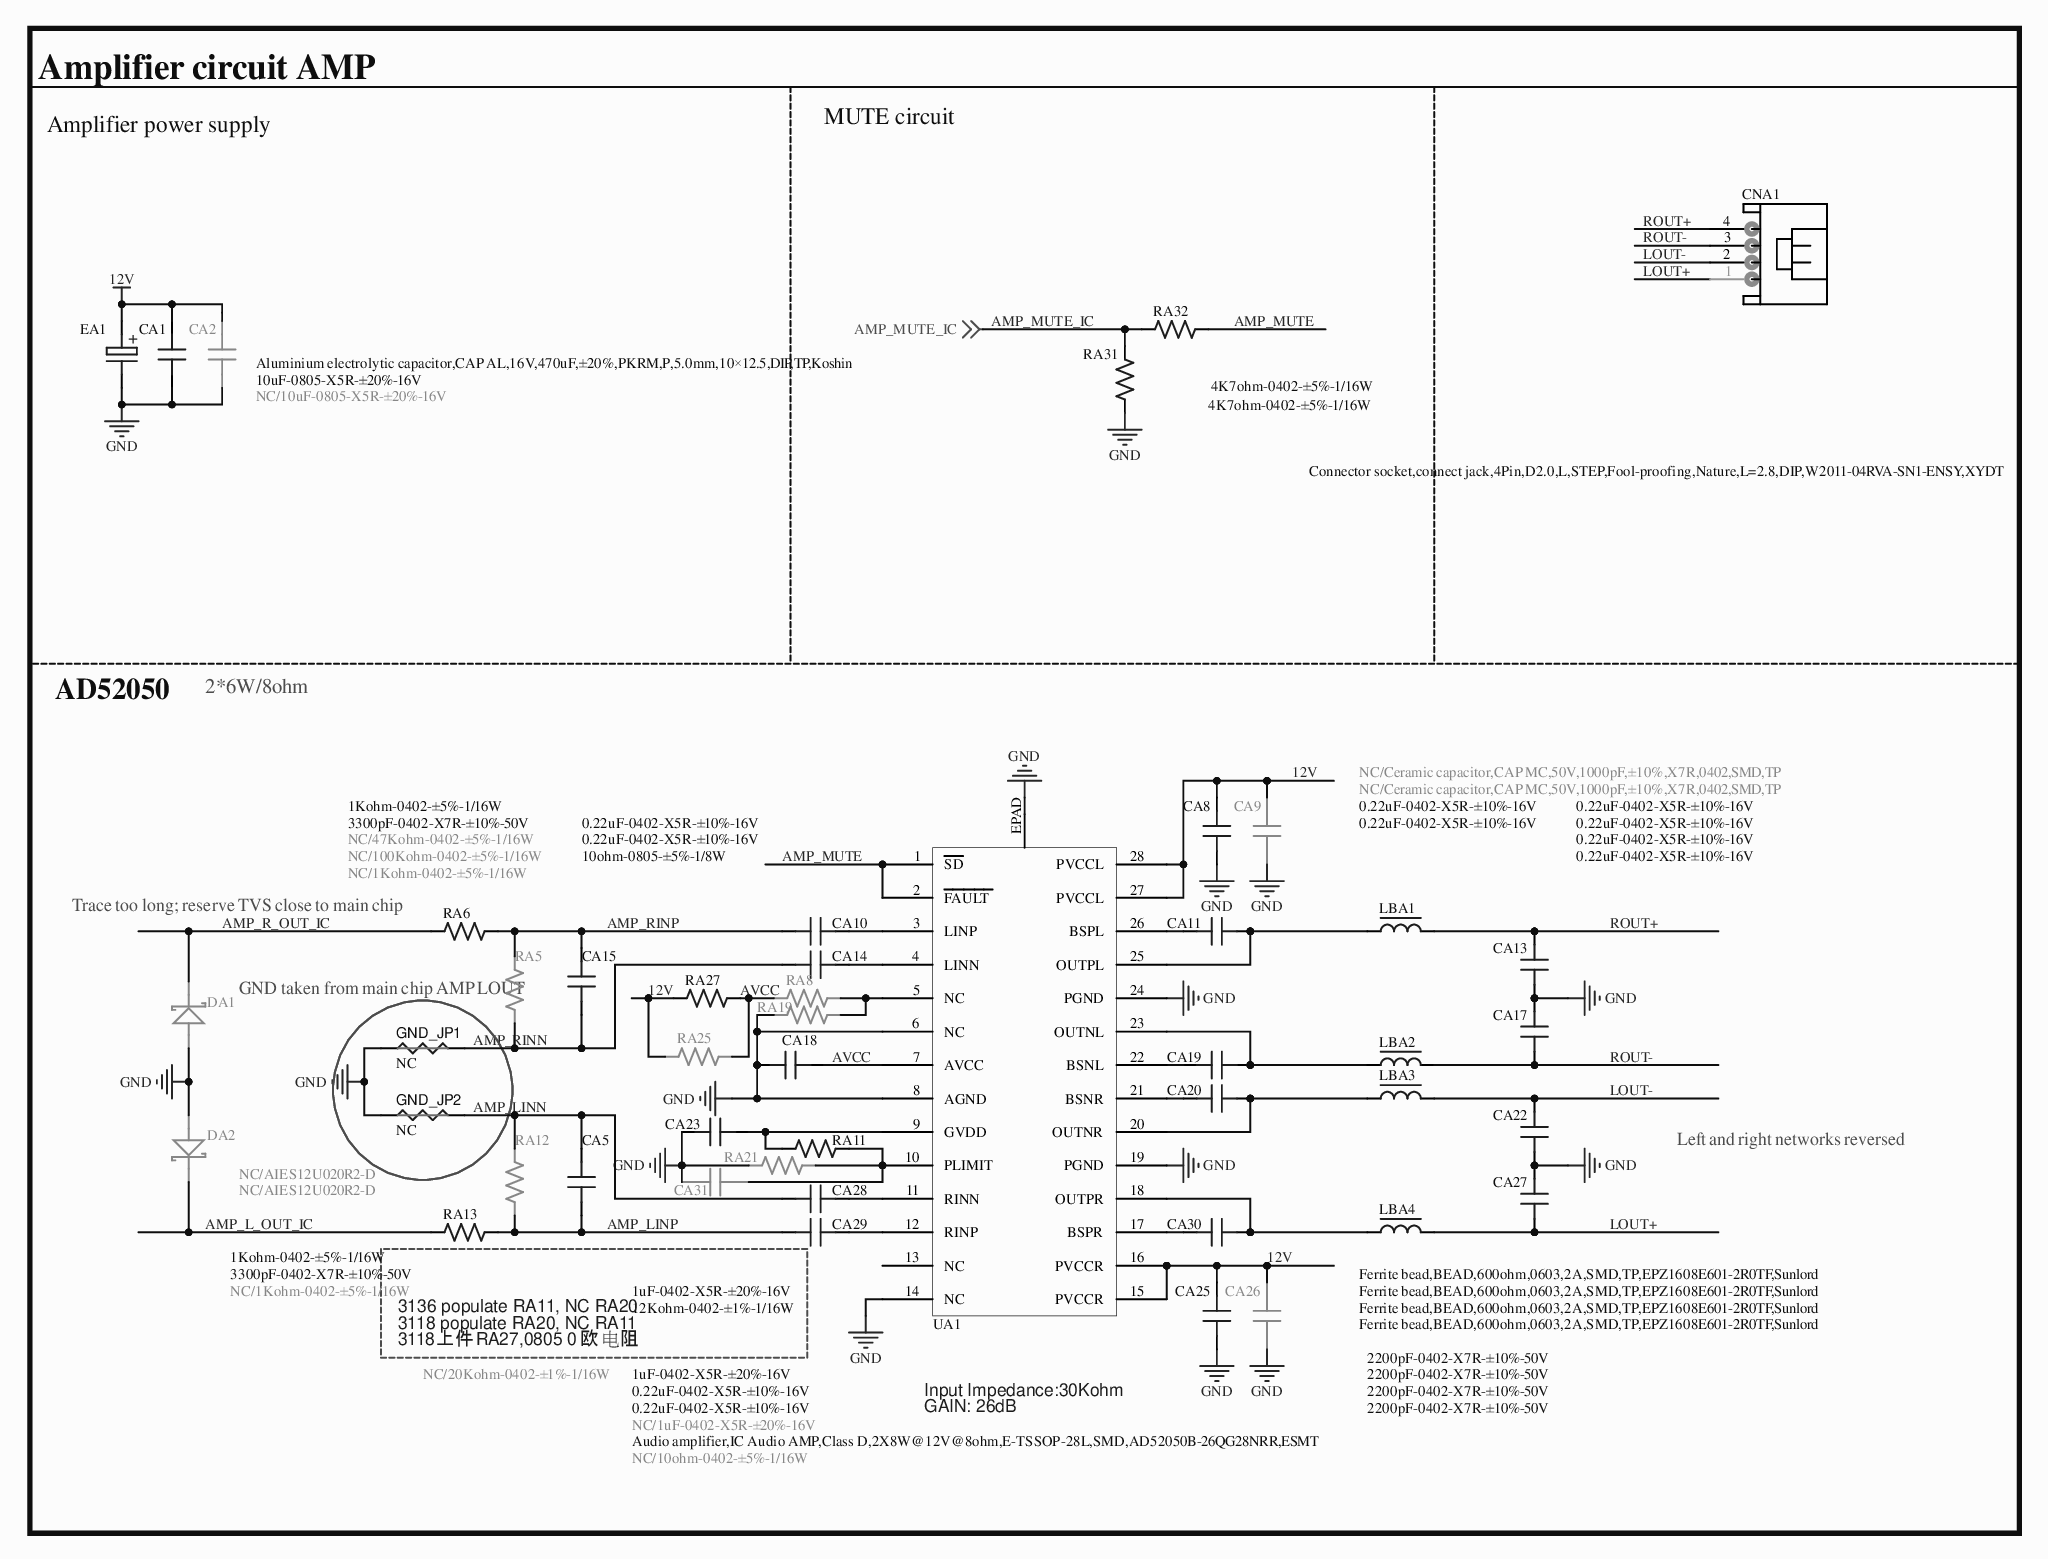
[diagram p0: MISC84395-16.SchDoc]
# Altium project MISC84395-37.PrjPCB (part 10 of 13)

## Sheet MISC84395-16.SchDoc
size 393 x 342 mm

### Parts
CA1  10uF-0805-X5R-±20%-16V  [C0805]
CA2  NC/10uF-0805-X5R-±20%-16V  [C0805]
CA5  3300pF-0402-X7R-±10%-50V  [C0402]
CA8  0.22uF-0402-X5R-±10%-16V  [C0402]
CA9  NC/Ceramic capacitor,CAP MC,50V,1000pF,±10%,X7R,0402,SMD,TP  [C0402]
CA10  0.22uF-0402-X5R-±10%-16V  [C0402]
CA11  0.22uF-0402-X5R-±10%-16V  [C0402]
CA13  2200pF-0402-X7R-±10%-50V  [C0402]
CA14  0.22uF-0402-X5R-±10%-16V  [C0402]
CA15  3300pF-0402-X7R-±10%-50V  [C0402]
CA17  2200pF-0402-X7R-±10%-50V  [C0402]
CA18  1uF-0402-X5R-±20%-16V  [C0402]
CA19  0.22uF-0402-X5R-±10%-16V  [C0402]
CA20  0.22uF-0402-X5R-±10%-16V  [C0402]
CA22  2200pF-0402-X7R-±10%-50V  [C0402]
CA23  1uF-0402-X5R-±20%-16V  [C0402]
CA25  0.22uF-0402-X5R-±10%-16V  [C0402]
CA26  NC/Ceramic capacitor,CAP MC,50V,1000pF,±10%,X7R,0402,SMD,TP  [C0402]
CA27  2200pF-0402-X7R-±10%-50V  [C0402]
CA28  0.22uF-0402-X5R-±10%-16V  [C0402]
CA29  0.22uF-0402-X5R-±10%-16V  [C0402]
CA30  0.22uF-0402-X5R-±10%-16V  [C0402]
CA31  NC/1uF-0402-X5R-±20%-16V  [C0402]
CNA1  Connector socket,connect jack,4Pin,D2.0,L,STEP,Fool-proofing,Nature,L=2.8,DIP,W2011-04RVA-SN1-ENSY,XYDT  [SIP4H/2.0D-6]
DA1  NC/AIES12U020R2-D  [DIODE-S0402]
DA2  NC/AIES12U020R2-D  [DIODE-S0402]
EA1  Aluminium electrolytic capacitor,CAP AL,16V,470uF,±20%,PKRM,P,5.0mm,10×12.5,DIP,TP,Koshin  [EC(10*12)-V-5]
GND_JP1  NC  [GND]
GND_JP2  NC  [GND]
LBA1  Ferrite bead,BEAD,600ohm,0603,2A,SMD,TP,EPZ1608E601-2R0TF,Sunlord  [L0603]
LBA2  Ferrite bead,BEAD,600ohm,0603,2A,SMD,TP,EPZ1608E601-2R0TF,Sunlord  [L0603]
LBA3  Ferrite bead,BEAD,600ohm,0603,2A,SMD,TP,EPZ1608E601-2R0TF,Sunlord  [L0603]
LBA4  Ferrite bead,BEAD,600ohm,0603,2A,SMD,TP,EPZ1608E601-2R0TF,Sunlord  [L0603]
RA5  NC/1Kohm-0402-±5%-1/16W  [R0402]
RA6  1Kohm-0402-±5%-1/16W  [R0402]
RA8  NC/100Kohm-0402-±5%-1/16W  [R0402]
RA11  12Kohm-0402-±1%-1/16W  [R0402]
RA12  NC/1Kohm-0402-±5%-1/16W  [R0402]
RA13  1Kohm-0402-±5%-1/16W  [R0402]
RA19  NC/47Kohm-0402-±5%-1/16W  [R0402]
RA21  NC/20Kohm-0402-±1%-1/16W  [R0402]
RA25  NC/10ohm-0402-±5%-1/16W  [R0402]
RA27  10ohm-0805-±5%-1/8W  [R0805]
RA31  4K7ohm-0402-±5%-1/16W  [R0402]
RA32  4K7ohm-0402-±5%-1/16W  [R0402]
UA1  Audio amplifier,IC Audio AMP,Class D,2X8W@12V@8ohm,E-TSSOP-28L,SMD,AD52050B-26QG28NRR,ESMT  [SOP28/0.65-7]

### Nets
12V: CA1.2 CA2.2 CA8.2 CA9.2 CA25.1 CA26.2 EA1.1 RA25.1 RA27.1 UA1.15(PVCCR) UA1.16(PVCCR) UA1.27(PVCCL) UA1.28(PVCCL)
GND: CA1.1 CA2.1 CA8.1 CA9.1 CA13.1 CA17.2 CA18.2 CA22.1 CA23.2 CA25.2 CA26.1 CA27.2 CA31.2 DA1.A DA2.A EA1.2 GND_JP1.JP_2K GND_JP2.JP_2K RA19.1 RA21.1 RA31.1 UA1.6(NC) UA1.8(AGND) UA1.14(NC) UA1.19(PGND) UA1.24(PGND) UA1.EPAD
AMP_L_OUT_IC: DA2.K RA13.1
AMP_LINN: CA5.2 CA28.2 GND_JP2.JP_1K RA12.2
AMP_LINP: CA5.1 CA29.2 RA12.1 RA13.2
AMP_MUTE: RA32.1 UA1.1(~{SD}) UA1.2(~{FAULT})
AMP_MUTE_IC: RA31.2 RA32.2 ; off-sheet AMP_MUTE_IC
AMP_R_OUT_IC: DA1.K RA6.1
AMP_RINN: CA14.2 CA15.1 GND_JP1.JP_1K RA5.1
AMP_RINP: CA10.2 CA15.2 RA5.2 RA6.2
AVCC: CA18.1 RA8.1 RA25.2 RA27.2 UA1.7(AVCC)
LOUT+: CA27.1 CNA1.1 LBA4.2
LOUT-: CA22.2 CNA1.2 LBA3.2
ROUT+: CA13.2 CNA1.4 LBA1.2
ROUT-: CA17.1 CNA1.3 LBA2.2
NetCA10_1: CA10.1 UA1.3(LINP)
NetCA11_1: CA11.1 LBA1.1 UA1.25(OUTPL)
NetCA11_2: CA11.2 UA1.26(BSPL)
NetCA14_1: CA14.1 UA1.4(LINN)
NetCA19_1: CA19.1 LBA2.1 UA1.23(OUTNL)
NetCA19_2: CA19.2 UA1.22(BSNL)
NetCA20_1: CA20.1 LBA3.1 UA1.20(OUTNR)
NetCA20_2: CA20.2 UA1.21(BSNR)
NetCA23_1: CA23.1 RA11.1 UA1.9(GVDD)
NetCA28_1: CA28.1 UA1.11(RINN)
NetCA29_1: CA29.1 UA1.12(RINP)
NetCA30_1: CA30.1 LBA4.1 UA1.18(OUTPR)
NetCA30_2: CA30.2 UA1.17(BSPR)
NetCA31_1: CA31.1 RA11.2 RA21.2 UA1.10(PLIMIT)
NetRA8_2: RA8.2 RA19.2 UA1.5(NC)

Not connected (* = marked no-connect by the designer): UA1 13(NC)*

### Notes on the sheet
- Amplifier circuit AMP
- Amplifier power supply
- MUTE circuit
- AD52050
- 2*6W/8ohm
- (near RA6) Trace too long; reserve TVS close to main chip
- (near RA5) GND taken from main chip AMP LOUT
- Left and right networks reversed
- 3136 populate RA11, NC RA20
- 3118 populate RA20, NC RA11
- 3118上件RA27,0805 0欧电阻
- GAIN: 26dB
- Input Impedance:30Kohm

### Library data of the parts
CA1 CA2 = 10uF-0805-X5R-±20%-16V-D
CA5 CA15 = 3300pF-0402-X7R-±10%-50V-D
CA8 CA18 CA23 CA25 CA31 = 1uF-0402-X5R-±20%-16V-D
CA9 CA26 = 1000pF-0402-X7R-±10%-50V-D
CA10 CA14 CA28 CA29 = 0.1uF-0402-X5R-±20%-16V-D
CA11 CA19 CA20 CA30 = 0.22uF-0402-X5R-±10%-16V-D
CA13 CA17 CA22 CA27 = 2200pF-0402-X7R-±10%-50V-D
CNA1 = XXX.XXX.0001726-DLMI: Connector socket,connect jack,4Pin,D2.0,L,SNAP,STEP,Nature,L=2.8mm,DIP,AMA-DLMI
DA1 DA2 = AIES12U020R2-D
EA1 = 470uF-16V±20%-10×12-105℃-编带-F=5.0-XL-DHAI
GND_JP1 GND_JP2 = GND: Manufacturer: Panasonic; Part Number: ERJ3GEYJ473V; Right: 20; Bottom: 30; CLASS: Discrete; Comments: Digikey
LBA1-LBA4 = 004.004.0000327-D: Ferrite bead,BEAD,120ohm,0603,600mA,SMD,TP,FCM1608KF-121T06-D
RA5 RA6 RA12 RA13 = 1Kohm-0402-±5%-1/16W-D
RA8 = 100Kohm-0402-±5%-1/16W-D
RA11 = 12Kohm-0402-±5%-1/16W-D
RA19 = 47Kohm-0402-±5%-1/16W-D
RA21 = 20Kohm-0402-±1%-1/16W-D
RA25 = 10ohm-0402-±5%-1/16W-D
RA27 = 10ohm-0805-±5%-1/8W-D
RA31 = 4K7ohm-0402-±5%-1/16W-D
RA32 = 4k7ohm-0402-±5%-1/16W-D
UA1 = 004.012.0000275-D: Audio amplifier,IC Audio AMP,Class D,2X8W@12V@8ohm,E-TSSOP-28L,SMD,AD52050B-26QG28NRR,ESMT-D

## Sheet MISC84395-17.SchDoc
size 381 x 292 mm
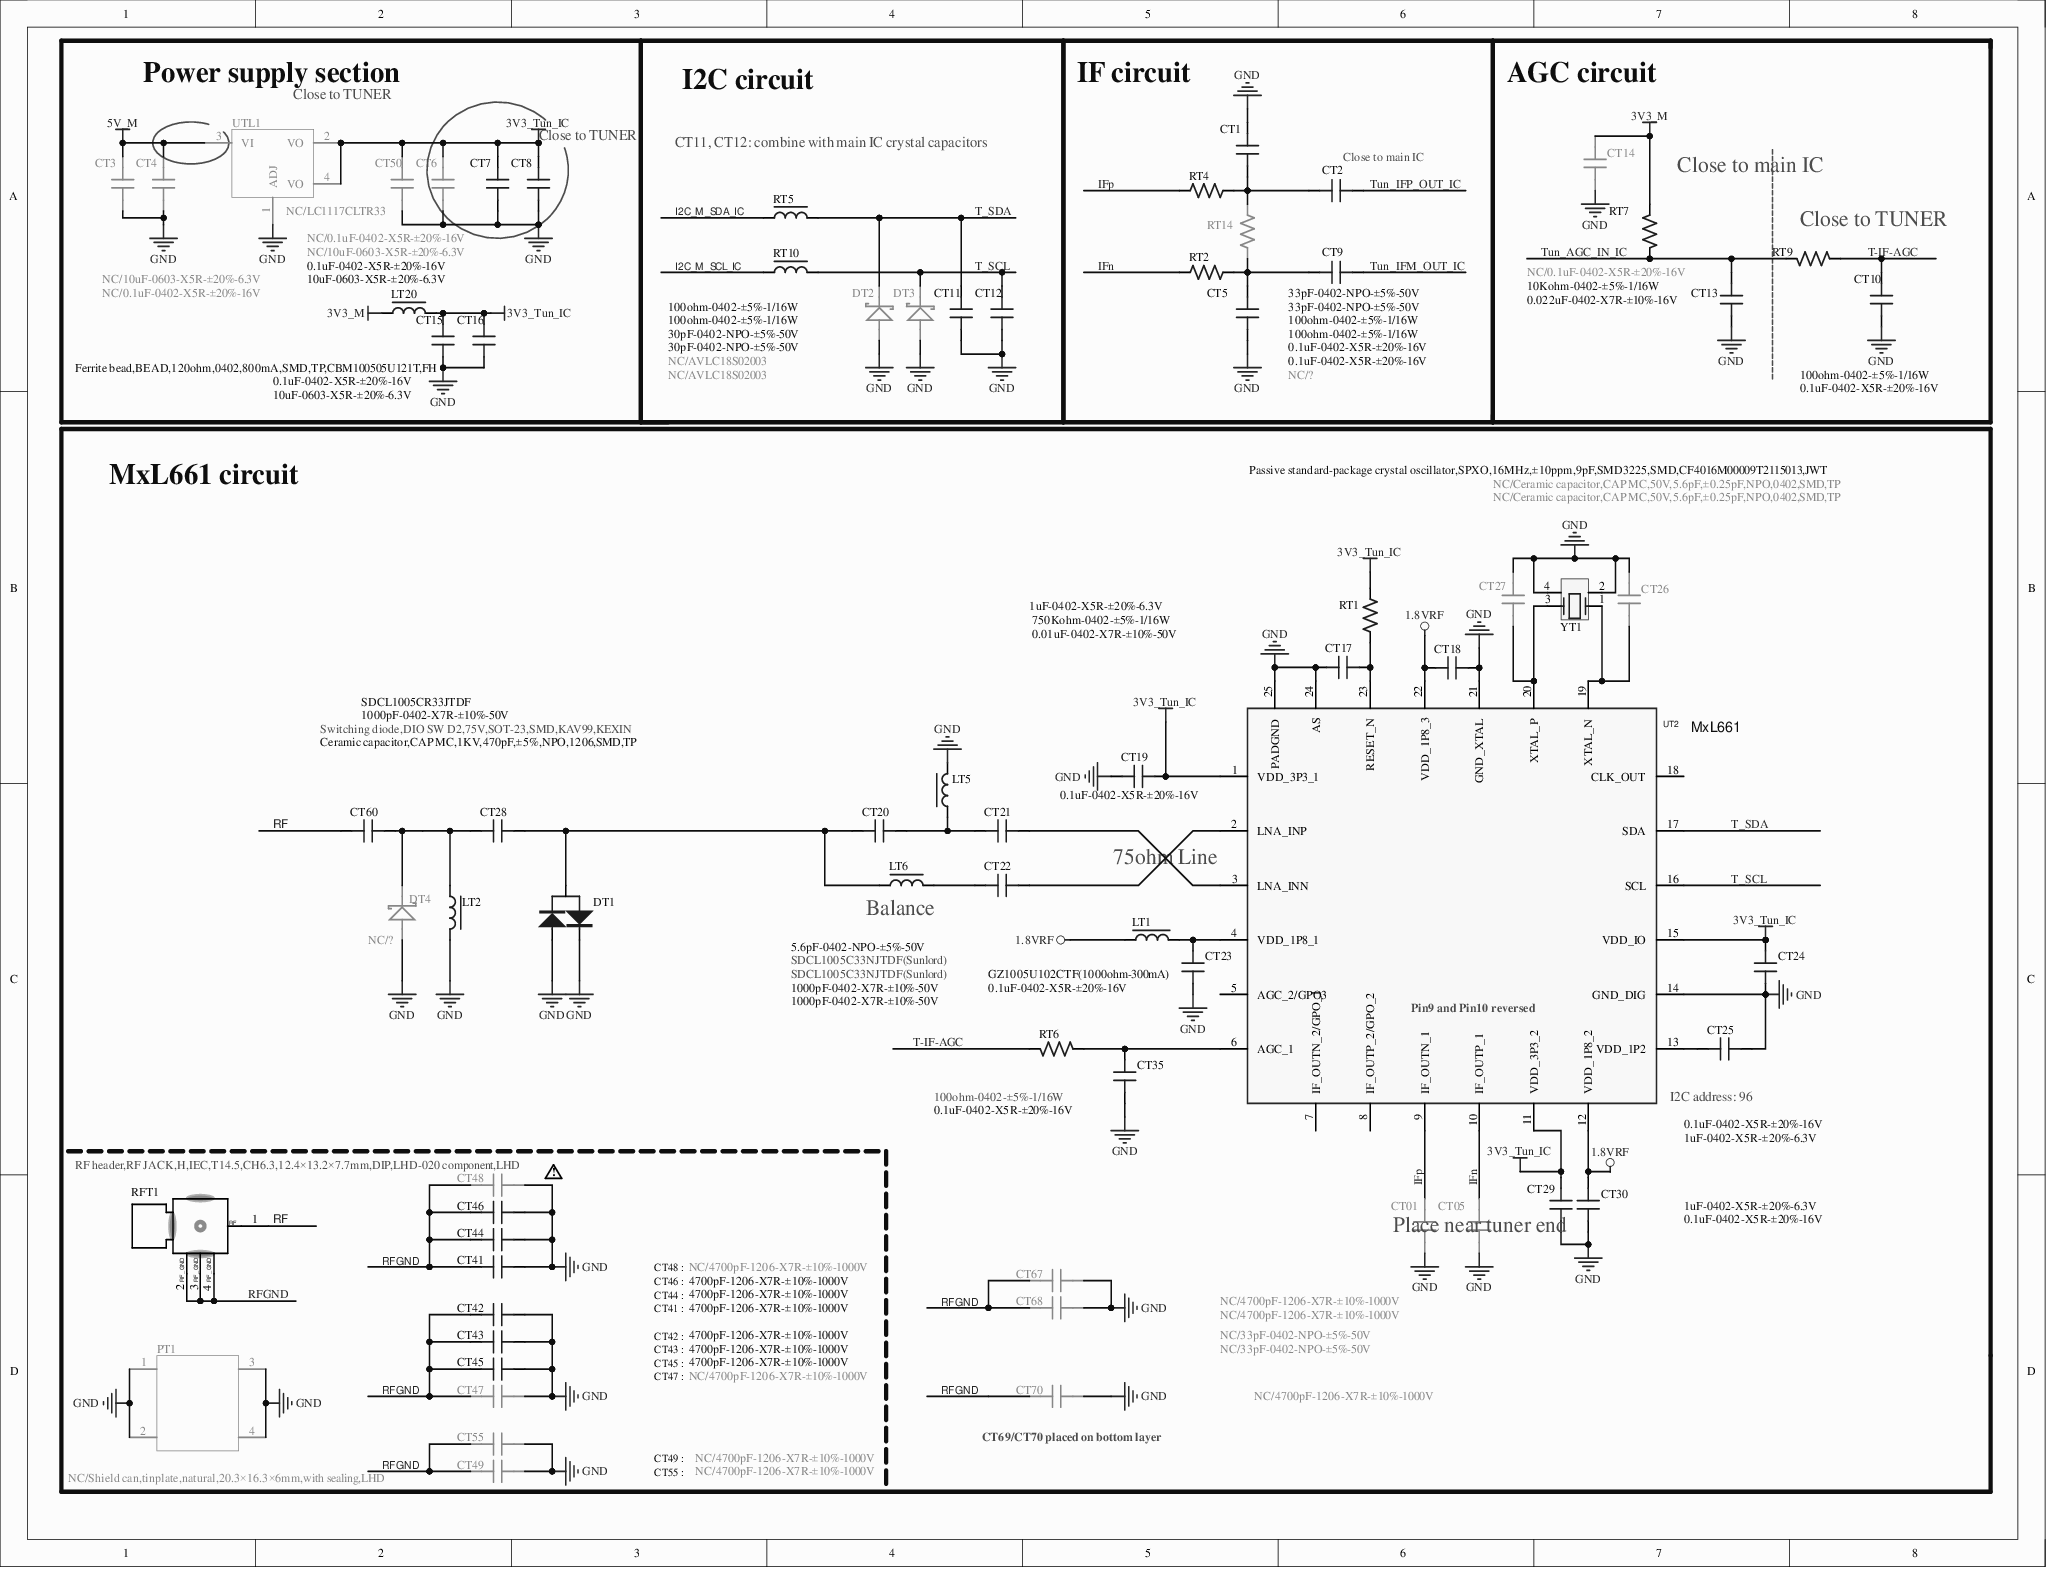
[diagram p1: MISC84395-17.SchDoc]

### Parts
CT1  33pF-0402-NPO-±5%-50V  [C0402]
CT01  NC/33pF-0402-NPO-±5%-50V  [C0402]
CT2  0.1uF-0402-X5R-±20%-16V  [C0402]
CT3  NC/10uF-0603-X5R-±20%-6.3V  [C0603]
CT4  NC/0.1uF-0402-X5R-±20%-16V  [C0402]
CT5  33pF-0402-NPO-±5%-50V  [C0402]
CT05  NC/33pF-0402-NPO-±5%-50V  [C0402]
CT6  NC/0.1uF-0402-X5R-±20%-16V  [C0402]
CT7  0.1uF-0402-X5R-±20%-16V  [C0402]
CT8  10uF-0603-X5R-±20%-6.3V  [C0603]
CT9  0.1uF-0402-X5R-±20%-16V  [C0402]
CT10  0.1uF-0402-X5R-±20%-16V  [C0402]
CT11  30pF-0402-NPO-±5%-50V  [C0402]
CT12  30pF-0402-NPO-±5%-50V  [C0402]
CT13  0.022uF-0402-X7R-±10%-16V  [C0402]
CT14  NC/0.1uF-0402-X5R-±20%-16V  [C0402]
CT15  10uF-0603-X5R-±20%-6.3V  [C0603]
CT16  0.1uF-0402-X5R-±20%-16V  [C0402]
CT17  1uF-0402-X5R-±20%-6.3V  [C0402]
CT18  0.01uF-0402-X7R-±10%-50V  [C0402]
CT19  0.1uF-0402-X5R-±20%-16V  [C0402]
CT20  5.6pF-0402-NPO-±5%-50V  [C0402]
CT21  1000pF-0402-X7R-±10%-50V  [C0402]
CT22  1000pF-0402-X7R-±10%-50V  [C0402]
CT23  0.1uF-0402-X5R-±20%-16V  [C0402]
CT24  0.1uF-0402-X5R-±20%-16V  [C0402]
CT25  1uF-0402-X5R-±20%-6.3V  [C0402]
CT26  NC/Ceramic capacitor,CAP MC,50V,5.6pF,±0.25pF,NPO,0402,SMD,TP  [C0402]
CT27  NC/Ceramic capacitor,CAP MC,50V,5.6pF,±0.25pF,NPO,0402,SMD,TP  [C0402]
CT28  1000pF-0402-X7R-±10%-50V  [C0402]
CT29  0.1uF-0402-X5R-±20%-16V  [C0402]
CT30  1uF-0402-X5R-±20%-6.3V  [C0402]
CT35  0.1uF-0402-X5R-±20%-16V  [C0402]
CT41  4700pF-1206-X7R-±10%-1000V  [C1206]
CT42  4700pF-1206-X7R-±10%-1000V  [C1206]
CT43  4700pF-1206-X7R-±10%-1000V  [C1206]
CT44  4700pF-1206-X7R-±10%-1000V  [C1206]
CT45  4700pF-1206-X7R-±10%-1000V  [C1206]
CT46  4700pF-1206-X7R-±10%-1000V  [C1206]
CT47  NC/4700pF-1206-X7R-±10%-1000V  [C1206]
CT48  NC/4700pF-1206-X7R-±10%-1000V  [C1206]
CT49  NC/4700pF-1206-X7R-±10%-1000V  [C1206]
CT50  NC/10uF-0603-X5R-±20%-6.3V  [C0603]
CT55  NC/4700pF-1206-X7R-±10%-1000V  [C1206]
CT60  Ceramic capacitor,CAP MC,1KV,470pF,±5%,NPO,1206,SMD,TP  [C1206]
CT67  NC/4700pF-1206-X7R-±10%-1000V  [C1206]
CT68  NC/4700pF-1206-X7R-±10%-1000V  [C1206]
CT70  NC/4700pF-1206-X7R-±10%-1000V  [C1206]
DT1  Switching diode,DIO SW D2,75V,SOT-23,SMD,KAV99,KEXIN  [SO-23]
DT2  NC/AVLC18S02003  [DIODE-S0402]
DT3  NC/AVLC18S02003  [DIODE-S0402]
DT4  NC/?  [DIODE-S0402]
LT1  GZ1005U102CTF(1000ohm-300mA)  [L0402]
LT2  SDCL1005CR33JTDF  [L0402]
LT5  SDCL1005C33NJTDF(Sunlord)  [L0402]
LT6  SDCL1005C33NJTDF(Sunlord)  [L0402]
LT20  Ferrite bead,BEAD,120ohm,0402,800mA,SMD,TP,CBM100505U121T,FH  [L0402]
PT1  NC/Shield can,tinplate,natural,20.3×16.3×6mm,with sealing,LHD  [SHIELD(16*20*6)]
RFT1  RF header,RF JACK,H,IEC,T14.5,CH6.3,12.4×13.2×7.7mm,DIP,LHD-020 component,LHD  [ANT-IEC14.5-H-4]
RT1  750Kohm-0402-±5%-1/16W  [R0402]
RT2  100ohm-0402-±5%-1/16W  [R0402]
RT4  100ohm-0402-±5%-1/16W  [R0402]
RT5  100ohm-0402-±5%-1/16W  [L0402]
RT6  100ohm-0402-±5%-1/16W  [R0402]
RT7  10Kohm-0402-±5%-1/16W  [R0402]
RT9  100ohm-0402-±5%-1/16W  [R0402]
RT10  100ohm-0402-±5%-1/16W  [L0402]
RT14  NC/?  [R0402]
UT2  MxL661  [QFN24/0.5-1]
UTL1  NC/LC1117CLTR33  [SOT-223]
YT1  Passive standard-package crystal oscillator,SPXO,16MHz,±10ppm,9pF,SMD3225,SMD,CF4016M00009T2115013,JWT  [XTAL-S-3]

### Blocks framed on the sheet
I2C circuit: CT11 CT12 DT2 DT3 RT5 RT10
MxL661 circuit: CT01 CT05 CT17-CT30 CT35 CT41-CT49 CT55 CT60 CT67 CT68 CT70 DT1 DT4 LT1 LT2 LT5 LT6 PT1 RFT1 RT1 RT6 UT2 YT1

### Nets
1.8VRF: CT18.1 CT30.2 LT1.1 UT2.12(VDD_1P8_2) UT2.22(VDD_1P8_3)
3V3_M: CT14.1 LT20.1 RT7.1
3V3_Tun_IC: CT6.2 CT7.2 CT8.1 CT15.2 CT16.2 CT19.1 CT24.1 CT29.2 CT50.2 LT20.2 RT1.2 UT2.1(VDD_3P3_1) UT2.11(VDD_3P3_2) UT2.15(VDD_IO) UTL1.2(VO) UTL1.4(VO)
5V_M: CT3.2 CT4.1 UTL1.3(VI)
GND: CT01.1 CT1.2 CT3.1 CT4.2 CT5.1 CT05.1 CT6.1 CT7.1 CT8.2 CT10.1 CT11.1 CT12.1 CT13.1 CT14.2 CT15.1 CT16.1 CT17.1 CT18.2 CT19.2 CT23.2 CT24.2 CT25.1 CT26.1 CT27.1 CT29.1 CT30.1 CT35.2 CT41.1 CT42.1 CT43.1 CT44.1 CT45.1 CT46.1 CT47.1 CT48.1 CT49.1 CT50.1 CT55.1 CT67.1 CT68.1 CT70.1 DT1.1 DT1.3 DT2.A DT3.A DT4.A LT2.2 LT5.1 PT1.1 PT1.2 PT1.3 PT1.4 UT2.14(GND_DIG) UT2.21(GND_XTAL) UT2.24(AS) UT2.25(PADGND) UTL1.1(ADJ) YT1.2(G) YT1.4
I2C_M_SCL_IC: RT10.1
I2C_M_SDA_IC: RT5.1
IFn: CT05.2 RT2.1 UT2.10(IF_OUTP_1)
IFp: CT01.2 RT4.1 UT2.9(IF_OUTN_1)
RF: CT60.1 RFT1.1
RFGND: CT41.2 CT42.2 CT43.2 CT44.2 CT45.2 CT46.2 CT47.2 CT48.2 CT49.2 CT55.2 CT67.2 CT68.2 CT70.2 RFT1.2 RFT1.3 RFT1.4
T-IF-AGC: CT10.2 RT6.2 RT9.1
T_SCL: CT12.2 DT3.K RT10.2 UT2.16(SCL)
T_SDA: CT11.2 DT2.K RT5.2 UT2.17(SDA)
Tun_AGC_IN_IC: CT13.2 RT7.2 RT9.2
Tun_IFM_OUT_IC: CT9.2
Tun_IFP_OUT_IC: CT2.2
NetCT1_1: CT1.1 CT2.1 RT4.2 RT14.2
NetCT5_2: CT5.2 CT9.1 RT2.2 RT14.1
NetCT17_2: CT17.2 RT1.1 UT2.23(RESET_N)
NetCT20_1: CT20.1 CT28.1 DT1.2 LT6.2
NetCT20_2: CT20.2 CT21.1 LT5.2
NetCT21_2: CT21.2 UT2.3(LNA_INN)
NetCT22_1: CT22.1 LT6.1
NetCT22_2: CT22.2 UT2.2(LNA_INP)
NetCT23_1: CT23.1 LT1.2 UT2.4(VDD_1P8_1)
NetCT25_2: CT25.2 UT2.13(VDD_1P2)
NetCT26_2: CT26.2 UT2.19(XTAL_N) YT1.1
NetCT27_2: CT27.2 UT2.20(XTAL_P) YT1.3
NetCT28_2: CT28.2 CT60.2 DT4.K LT2.1
NetCT35_1: CT35.1 RT6.1 UT2.6(AGC_1)

Not connected (* = marked no-connect by the designer): UT2 5(AGC_2/GPO3)* 7(IF_OUTN_2/GPO_1)* 8(IF_OUTP_2/GPO_2)* 18(CLK_OUT)*

### Notes on the sheet
- Power supply section
- (near UTL1) Close to TUNER
- (near CT1) IF circuit
- AGC circuit
- (near CT8) Close to TUNER
- CT11, CT12: combine with main IC crystal capacitors
- (near CT2) Close to main IC
- (near RT7) Close to main IC
- (near RT9) Close to TUNER
- (near LT6) Balance
- (near UT2) 75ohm Line
- (near UT2) Pin9 and Pin10 reversed
- (near UT2) I2C address: 96
- !
- Place near tuner end
- CT41 :
- CT44 :
- CT46 :
- CT48 :
- CT42 :
- CT43 :
- CT45 :
- CT47 :
- CT49 :
- (near CT70) CT69/CT70 placed on bottom layer
- CT55 :

### Library data of the parts
CT1 CT01 CT5 CT05 CT11 CT12 = 33pF-0402-NPO-±5%-50V-D
CT2 CT4 CT6 CT7 CT9 CT10 CT14 CT16 CT19 CT23 CT24 CT29 CT35 = 0.1uF-0402-Y5V-+80%-20%-16V-D
CT3 CT8 CT15 CT50 = 10uF-0603-X5R-±20%-6.3V-D
CT13 = 0.022uF-0402-X7R-±10%-16V-D
CT17 CT25 CT30 = 1uF-0402-X5R-±20%-6.3V-D
CT18 = 0.01uF-0402-X7R-±10%-50V-D
CT20 = 5.6pF-0402-NPO-±5%-50V-D
CT21 CT22 CT28 = 1000pF-0402-X7R-±10%-50V-D
CT26 CT27 = 22pF-0402-NPO-±5%-50V-D
CT41-CT49 CT55 CT67 CT68 CT70 = 1000pF-1206-X7R-±20%-2000V-D
CT60 = 4700pF-1206-X7R-±10%-1000V-D
DT1 = BAV99-BR-D
DT2 DT3 = AVLC18S02003-D
DT4 = AIES12U020R2-D
LT1 = MGHB1005S102T-LF-D
LT2 = SDCL1005CR33JTDF-D
LT5 LT6 = SDCL1005C33NJTDF(顺络) -D
LT20 = FCM1005KF-121T06(120ohm-500mA)-D
PT1 = 004.040.0000768-DMI: Shield can,tinplate,natural,20.3×16.3×6mm,with sealing,LHD-DMI
RFT1 = RF头,RF JACK,H,IEC,T14.5,CH6.3,12.4×13.2×7.7mm,DIP,LHD-020组件,LHD-DLMI: T-IEC-6.3mm-#-#
RT1 = 750Kohm-0402-±5%-1/16W-D
RT2 RT4 = 004.002.0000568-D: Thick film resistor,RES,1/16W,100ohm,±5%,0402,SMD-D
RT5 RT10 = 300ohm-0402-±25%-D
RT6 = 100ohm-0402-±5%-1/16W-D
RT7 RT9 = 10Kohm-0402-±5%-1/16W-D
RT14 = 0ohm-0402-±5%-1/16W-D
UT2 = MxL661-D: MFR PN: EN4020-B0; MFR: Entropic; ENTROPIC PN: 15-4000-0021; DESC: IC,  EN4020-B0,  Multi-Standard Tuner
UTL1 = LC1117CLTR33-D
YT1 = 32MHz-±10PPM-12PF-SMD3225-JWT-D